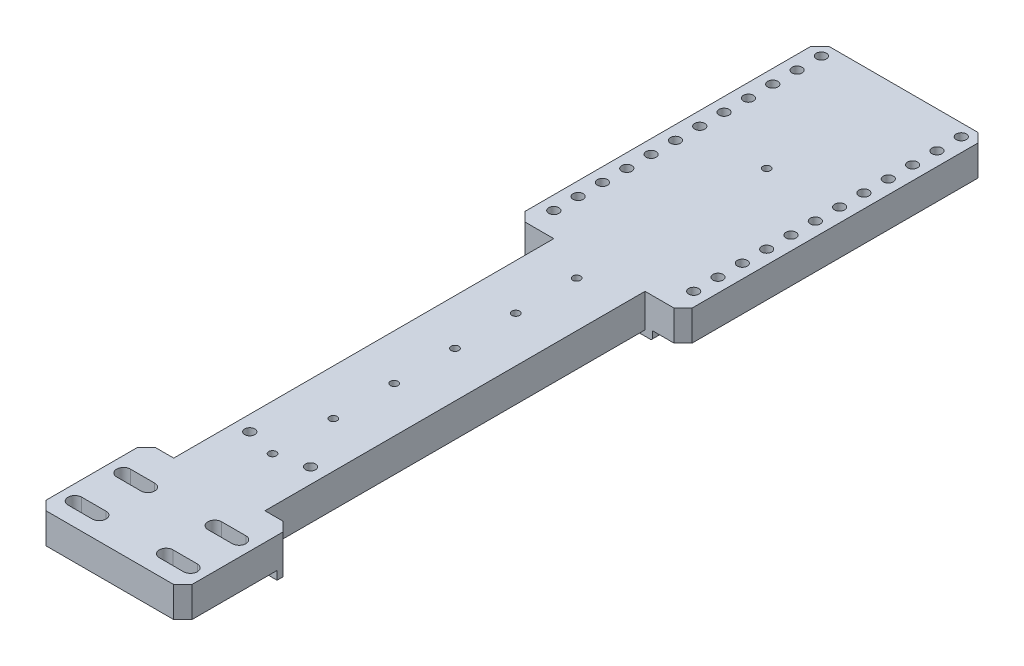
from build123d import *

# Parameters (mm, degrees)
SKETCH1_W             = 55
SKETCH1_H             = 265
BOSS_EXTRUDE1_DEPTH   = 10
SKETCH2_W             = 35
SKETCH2_H             = 100
BOSS_EXTRUDE2_DEPTH   = 2.8
SKETCH4_W             = 12.5
SKETCH4_H             = 130
CUT_EXTRUDE2_DEPTH    = 136.927701371
CUT_EXTRUDE3_DEPTH    = 38
CHAMFER2_SIZE         = 0.5
CHAMFER3_SIZE         = 3
LPATTERN1_COUNT       = 12
LPATTERN1_PITCH       = 8
SKETCH9_W             = 10.5
SKETCH9_H             = 130
BOSS_EXTRUDE3_DEPTH   = 1
SKETCH10_W            = 12.5
SKETCH10_H            = 12.8
BOSS_EXTRUDE4_DEPTH   = 5
CUT_EXTRUDE4_START    = -2.8
SKETCH11_R            = 1
CUT_EXTRUDE4_DEPTH    = 2.8
M3_TAPPED_HOLE1_D     = 2.5
LPATTERN2_COUNT       = 6
LPATTERN2_PITCH       = 20
SKETCH15_W            = 10.5
SKETCH15_H            = 5
BOSS_EXTRUDE5_DEPTH   = 1.8
M4_TAPPED_HOLE2_D     = 3.3
SKETCH20_W            = 55
SKETCH20_H            = 4
CUT_EXTRUDE6_DEPTH    = 136.927701371
SKETCH21_W            = 3.5
SKETCH21_H            = 36
CUT_EXTRUDE7_DEPTH    = 136.927701371
CHAMFER4_SIZE         = 3
M3_TAPPED_HOLE2_D     = 2.5
M3_TAPPED_HOLE2_DEPTH = 7.5
M3_TAPPED_HOLE2_TIP   = 0.751075774


with BuildPart() as part:
    # Sketch1 → Boss-Extrude1 (new body)
    with BuildSketch(Plane(origin=(0, 0, 0), x_dir=(1, 0, 0), z_dir=(0, 1, 0))):
        Rectangle(SKETCH1_W, SKETCH1_H)
    extrude(amount=BOSS_EXTRUDE1_DEPTH)

    # Sketch2 → Boss-Extrude2 (add)
    with BuildSketch(Plane.XZ):
        with Locations((0, -82.5)):
            Rectangle(SKETCH2_W, SKETCH2_H)
    extrude(amount=BOSS_EXTRUDE2_DEPTH)

    # Sketch4 → Cut-Extrude2 (cut, through all)
    with BuildSketch(Plane.XZ.offset(2.8)):
        with Locations((-21.25, 32.5)):
            Rectangle(SKETCH4_W, SKETCH4_H)
        with Locations((21.25, 32.5)):
            Rectangle(SKETCH4_W, SKETCH4_H)
    extrude(amount=-CUT_EXTRUDE2_DEPTH, mode=Mode.SUBTRACT)

    # Sketch5 → Cut-Extrude3 (cut)
    with BuildSketch(Plane(origin=(0, 10, 0), x_dir=(1, 0, 0), z_dir=(0, 1, 0))):
        with BuildLine():
            Line((-19, -123.25), (-11, -123.25))
            ThreePointArc((-11, -123.25), (-8.75, -121), (-11, -118.75))
            Line((-11, -118.75), (-19, -118.75))
            ThreePointArc((-19, -118.75), (-21.25, -121), (-19, -123.25))
        make_face()
        with BuildLine():
            Line((19, -102.75), (11, -102.75))
            ThreePointArc((11, -102.75), (8.75, -105), (11, -107.25))
            Line((11, -107.25), (19, -107.25))
            ThreePointArc((19, -107.25), (21.25, -105), (19, -102.75))
        make_face()
        with BuildLine():
            Line((19, -123.25), (11, -123.25))
            ThreePointArc((11, -123.25), (8.75, -121), (11, -118.75))
            Line((11, -118.75), (19, -118.75))
            ThreePointArc((19, -118.75), (21.25, -121), (19, -123.25))
        make_face()
        with BuildLine():
            Line((-19, -102.75), (-11, -102.75))
            ThreePointArc((-11, -102.75), (-8.75, -105), (-11, -107.25))
            Line((-11, -107.25), (-19, -107.25))
            ThreePointArc((-19, -107.25), (-21.25, -105), (-19, -102.75))
        make_face()
    extrude(amount=-CUT_EXTRUDE3_DEPTH, mode=Mode.SUBTRACT)

    # Chamfer2
    chamfer2_edges = [part.edges().sort_by_distance(p)[0] for p in [
        (17.5, -2.8, -82.5),
        (-17.5, -2.8, -82.5),
    ]]
    chamfer(chamfer2_edges, length=CHAMFER2_SIZE)

    # Chamfer3
    chamfer3_edges = [part.edges().sort_by_distance(p)[0] for p in [
        (-27.5, 5, -132.5),
        (27.5, 5, -132.5),
        (27.5, 5, -32.5),
        (-27.5, 5, -32.5),
    ]]
    chamfer(chamfer3_edges, length=CHAMFER3_SIZE)

    # Sketch7 → M4 Tapped Hole1 (revolve, cut)
    with BuildSketch(Plane(origin=(-23, 0, -128.5), x_dir=(0, 0, -1), z_dir=(1, 0, 0))):
        Polygon((0, 0), (0, 11.091420021), (1.65, 10.1), (1.65, 0), align=None)
    m4_tapped_hole1 = revolve(axis=Axis((-23, -6.35, -128.5), (0, 1, 0)), mode=Mode.SUBTRACT)

    # Mirror1: M4 Tapped Hole1 across plane
    add(m4_tapped_hole1.mirror(Plane(origin=(0, 0, 0), x_dir=(0, 0, 1), z_dir=(1, 0, 0))), mode=Mode.SUBTRACT)

    # LPattern1: M4 Tapped Hole1 ×12
    with Locations(*[(0, 0, i * LPATTERN1_PITCH) for i in range(1, LPATTERN1_COUNT)]):
        add(m4_tapped_hole1, mode=Mode.SUBTRACT)

    # LPattern1 copy 1 sketch → LPattern1 copy 1 (revolve, cut)
    with BuildSketch(Plane(origin=(23, 0, -120.5), x_dir=(0, 0, -1), z_dir=(-1, 0, 0))):
        Polygon((0, 0), (0, -11.091420021), (1.65, -10.1), (1.65, 0), align=None)
    revolve(axis=Axis((23, -6.35, -120.5), (0, -1, 0)), mode=Mode.SUBTRACT)

    # LPattern1 copy 2 sketch → LPattern1 copy 2 (revolve, cut)
    with BuildSketch(Plane(origin=(23, 0, -112.5), x_dir=(0, 0, -1), z_dir=(-1, 0, 0))):
        Polygon((0, 0), (0, -11.091420021), (1.65, -10.1), (1.65, 0), align=None)
    revolve(axis=Axis((23, -6.35, -112.5), (0, -1, 0)), mode=Mode.SUBTRACT)

    # LPattern1 copy 3 sketch → LPattern1 copy 3 (revolve, cut)
    with BuildSketch(Plane(origin=(23, 0, -104.5), x_dir=(0, 0, -1), z_dir=(-1, 0, 0))):
        Polygon((0, 0), (0, -11.091420021), (1.65, -10.1), (1.65, 0), align=None)
    revolve(axis=Axis((23, -6.35, -104.5), (0, -1, 0)), mode=Mode.SUBTRACT)

    # LPattern1 copy 4 sketch → LPattern1 copy 4 (revolve, cut)
    with BuildSketch(Plane(origin=(23, 0, -96.5), x_dir=(0, 0, -1), z_dir=(-1, 0, 0))):
        Polygon((0, 0), (0, -11.091420021), (1.65, -10.1), (1.65, 0), align=None)
    revolve(axis=Axis((23, -6.35, -96.5), (0, -1, 0)), mode=Mode.SUBTRACT)

    # LPattern1 copy 5 sketch → LPattern1 copy 5 (revolve, cut)
    with BuildSketch(Plane(origin=(23, 0, -88.5), x_dir=(0, 0, -1), z_dir=(-1, 0, 0))):
        Polygon((0, 0), (0, -11.091420021), (1.65, -10.1), (1.65, 0), align=None)
    revolve(axis=Axis((23, -6.35, -88.5), (0, -1, 0)), mode=Mode.SUBTRACT)

    # LPattern1 copy 6 sketch → LPattern1 copy 6 (revolve, cut)
    with BuildSketch(Plane(origin=(23, 0, -80.5), x_dir=(0, 0, -1), z_dir=(-1, 0, 0))):
        Polygon((0, 0), (0, -11.091420021), (1.65, -10.1), (1.65, 0), align=None)
    revolve(axis=Axis((23, -6.35, -80.5), (0, -1, 0)), mode=Mode.SUBTRACT)

    # LPattern1 copy 7 sketch → LPattern1 copy 7 (revolve, cut)
    with BuildSketch(Plane(origin=(23, 0, -72.5), x_dir=(0, 0, -1), z_dir=(-1, 0, 0))):
        Polygon((0, 0), (0, -11.091420021), (1.65, -10.1), (1.65, 0), align=None)
    revolve(axis=Axis((23, -6.35, -72.5), (0, -1, 0)), mode=Mode.SUBTRACT)

    # LPattern1 copy 8 sketch → LPattern1 copy 8 (revolve, cut)
    with BuildSketch(Plane(origin=(23, 0, -64.5), x_dir=(0, 0, -1), z_dir=(-1, 0, 0))):
        Polygon((0, 0), (0, -11.091420021), (1.65, -10.1), (1.65, 0), align=None)
    revolve(axis=Axis((23, -6.35, -64.5), (0, -1, 0)), mode=Mode.SUBTRACT)

    # LPattern1 copy 9 sketch → LPattern1 copy 9 (revolve, cut)
    with BuildSketch(Plane(origin=(23, 0, -56.5), x_dir=(0, 0, -1), z_dir=(-1, 0, 0))):
        Polygon((0, 0), (0, -11.091420021), (1.65, -10.1), (1.65, 0), align=None)
    revolve(axis=Axis((23, -6.35, -56.5), (0, -1, 0)), mode=Mode.SUBTRACT)

    # LPattern1 copy 10 sketch → LPattern1 copy 10 (revolve, cut)
    with BuildSketch(Plane(origin=(23, 0, -48.5), x_dir=(0, 0, -1), z_dir=(-1, 0, 0))):
        Polygon((0, 0), (0, -11.091420021), (1.65, -10.1), (1.65, 0), align=None)
    revolve(axis=Axis((23, -6.35, -48.5), (0, -1, 0)), mode=Mode.SUBTRACT)

    # LPattern1 copy 11 sketch → LPattern1 copy 11 (revolve, cut)
    with BuildSketch(Plane(origin=(23, 0, -40.5), x_dir=(0, 0, -1), z_dir=(-1, 0, 0))):
        Polygon((0, 0), (0, -11.091420021), (1.65, -10.1), (1.65, 0), align=None)
    revolve(axis=Axis((23, -6.35, -40.5), (0, -1, 0)), mode=Mode.SUBTRACT)

    # Sketch9 → Boss-Extrude3 (add)
    with BuildSketch(Plane.XZ):
        with Locations((-9.75, 32.5)):
            Rectangle(SKETCH9_W, SKETCH9_H)
        with Locations((9.75, 32.5)):
            Rectangle(SKETCH9_W, SKETCH9_H)
    extrude(amount=BOSS_EXTRUDE3_DEPTH)

    # Sketch10 → Boss-Extrude4 (add)
    with BuildSketch(Plane(origin=(0, 0, 97.5), x_dir=(-1, 0, 0), z_dir=(0, 0, -1))):
        with Locations((21.25, 3.6)):
            Rectangle(SKETCH10_W, SKETCH10_H)
        with Locations((-21.25, 3.6)):
            Rectangle(SKETCH10_W, SKETCH10_H)
    extrude(amount=BOSS_EXTRUDE4_DEPTH)

    # Sketch11 → Cut-Extrude4 (cut)
    with BuildSketch(Plane.XZ.offset(2.8).offset(CUT_EXTRUDE4_START)):
        with Locations((4.5, -32.5)):
            Circle(SKETCH11_R)
        with Locations((-4.5, -32.5)):
            Circle(SKETCH11_R)
    extrude(amount=CUT_EXTRUDE4_DEPTH, mode=Mode.SUBTRACT)

    # M3 Tapped Hole1 (through all)
    with Locations(Plane(origin=(0, 0, 0), x_dir=(-1, 0, 0), z_dir=(0, -1, 0))):
        with Locations((0, 25)):
            m3_tapped_hole1 = Hole(M3_TAPPED_HOLE1_D / 2)

    # LPattern2: M3 Tapped Hole1 ×6
    with Locations(*[(0, 0, i * LPATTERN2_PITCH) for i in range(1, LPATTERN2_COUNT)]):
        add(m3_tapped_hole1, mode=Mode.SUBTRACT)

    # Sketch15 → Boss-Extrude5 (add)
    with BuildSketch(Plane.XZ.offset(1)):
        with Locations((-9.75, 95)):
            Rectangle(SKETCH15_W, SKETCH15_H)
        with Locations((9.75, 95)):
            Rectangle(SKETCH15_W, SKETCH15_H)
    extrude(amount=BOSS_EXTRUDE5_DEPTH)

    # M4 Tapped Hole2 (through all)
    with Locations(Plane(origin=(0, 10, 0), x_dir=(1, 0, 0), z_dir=(0, 1, 0))):
        with Locations((-10, -72.5), (10, -72.5)):
            Hole(M4_TAPPED_HOLE2_D / 2)

    # Sketch20 → Cut-Extrude6 (cut, through all)
    with BuildSketch(Plane(origin=(0, 10, 0), x_dir=(1, 0, 0), z_dir=(0, 1, 0))):
        with Locations((0, -130.5)):
            Rectangle(SKETCH20_W, SKETCH20_H)
    extrude(amount=-CUT_EXTRUDE6_DEPTH, mode=Mode.SUBTRACT)

    # Sketch21 → Cut-Extrude7 (cut, through all)
    with BuildSketch(Plane(origin=(0, 10, 0), x_dir=(1, 0, 0), z_dir=(0, 1, 0))):
        with Locations((-25.75, -110.5)):
            Rectangle(SKETCH21_W, SKETCH21_H)
        with Locations((25.75, -110.5)):
            Rectangle(SKETCH21_W, SKETCH21_H)
    extrude(amount=-CUT_EXTRUDE7_DEPTH, mode=Mode.SUBTRACT)

    # Chamfer4
    chamfer4_edges = [part.edges().sort_by_distance(p)[0] for p in [
        (-24, 5, 128.5),
        (-24, 3.6, 92.5),
        (24, 5, 128.5),
        (24, 3.6, 92.5),
    ]]
    chamfer(chamfer4_edges, length=CHAMFER4_SIZE)

    # M3 Tapped Hole2
    with Locations(Plane(origin=(0, 10, 0), x_dir=(1, 0, 0), z_dir=(0, 1, 0))):
        with Locations((0, 87.5)):
            Hole(M3_TAPPED_HOLE2_D / 2, depth=M3_TAPPED_HOLE2_DEPTH)
            with Locations((0, 0, -(M3_TAPPED_HOLE2_DEPTH + M3_TAPPED_HOLE2_TIP / 2))):  # 118° drill point
                Cone(0, M3_TAPPED_HOLE2_D / 2, M3_TAPPED_HOLE2_TIP, mode=Mode.SUBTRACT)


solid = part.part
